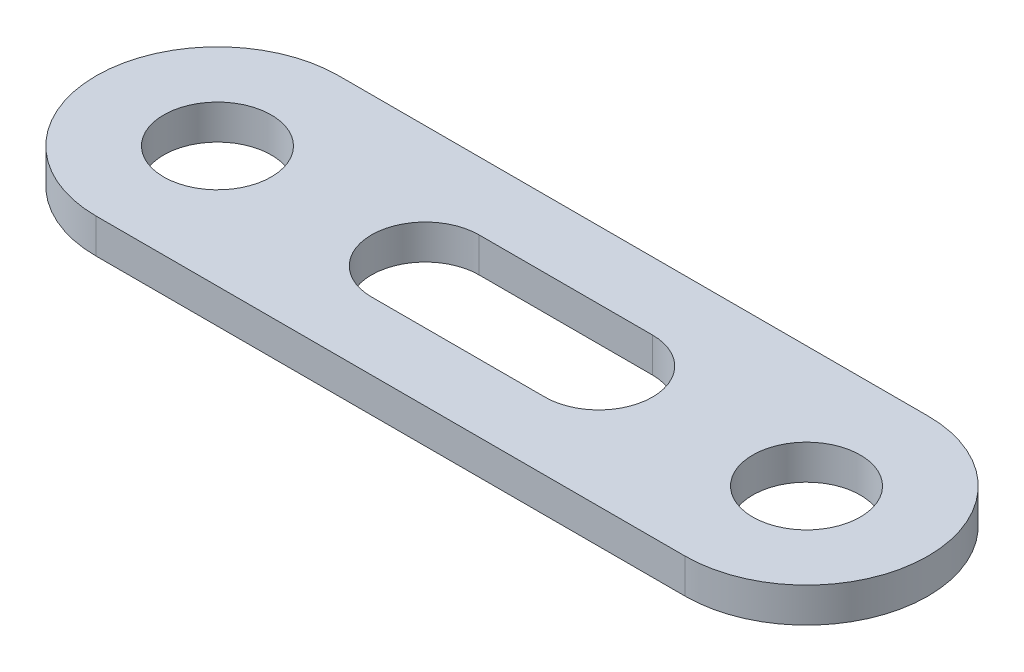
SolidWorks part; units mm, degrees
material "Thornel Mat VMA"
ref_plane "前视基准面" through (0, 0, 0) normal (0, 0, 1) x (1, 0, 0)
ref_plane "上视基准面" through (0, 0, 0) normal (0, 1, 0) x (1, 0, 0)
ref_plane "右视基准面" through (0, 0, 0) normal (1, 0, 0) x (0, 0, -1)
other "Configuration Table"
sketch "草图1" plane through (0, 0, 0) normal (0, 1, 0) x (1, 0, 0)
  line L0 (0, 0) -> (16.98, 0) construction
  line L1 (0, 3.5) -> (16.98, 3.5)
  line L2 (0, -3.5) -> (16.98, -3.5)
  line L3 (5.99, 0) -> (10.99, 0) construction
  line L4 (5.99, 1.55) -> (10.99, 1.55)
  line L5 (5.99, -1.55) -> (10.99, -1.55)
  circle A0 centre (0, 0) radius 1.55
  circle A1 centre (16.98, 0) radius 1.55
  circle A2 centre (16.98, 0) radius 3.5
  circle A3 centre (0, 0) radius 3.5
  arc A4 (5.99, 1.55) -> (5.99, -1.55) centre (5.99, 0) ccw
  arc A5 (10.99, -1.55) -> (10.99, 1.55) centre (10.99, 0) ccw
  point P13 (8.49, 0)
  dimension "D2" = 3.1
  dimension "D3" = 7
  dimension "D4" = 8.49
  dimension "D1" = 16.98
  dimension "D5" = 5
extrude "凸台-拉伸1" add sketch "草图1" along normal blind 1
